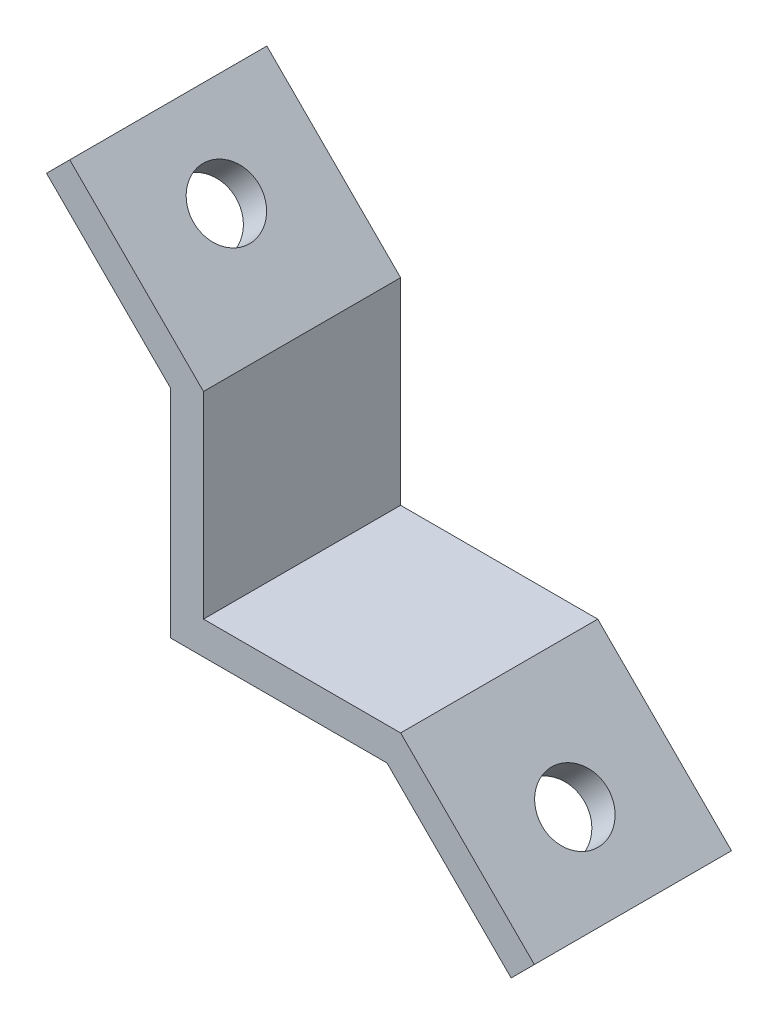
SolidWorks part; units mm, degrees
ref_plane "前视基准面" through (0, 0, 0) normal (0, 0, 1) x (1, 0, 0)
ref_plane "上视基准面" through (0, 0, 0) normal (0, 1, 0) x (1, 0, 0)
ref_plane "右视基准面" through (0, 0, 0) normal (1, 0, 0) x (0, 0, -1)
sketch "草图1" plane through (0, 0, 0) normal (0, 0, 1) x (1, 0, 0)
  line L0 (0, 0) -> (0, 60)
  line L1 (0, 60) -> (-10, 60)
  line L2 (-10, 60) -> (-10, -10)
  line L3 (-10, -10) -> (60, -10)
  line L4 (60, -10) -> (60, 0)
  line L5 (60, 0) -> (0, 0)
  dimension "D1" = 60
  dimension "D2" = 60
  dimension "D3" = 10
  dimension "D4" = 10
extrude "凸台-拉伸1" add sketch "草图1" along normal blind 60
sketch "草图2" plane through (0, 0, 0) normal (0, 0, 1) x (1, 0, 0)
  line L0 (0, 60) -> (-40.7107, 100.7107)
  line L1 (-40.7107, 100.7107) -> (-47.7817, 93.6396)
  line L2 (-47.7817, 93.6396) -> (-10, 55.8579)
  line L4 (-10, 55.8579) -> (-10, 60)
  line L5 (-10, 60) -> (0, 60)
  line L6 (60, 0) -> (100.7107, -40.7107)
  line L7 (100.7107, -40.7107) -> (93.6396, -47.7817)
  line L8 (93.6396, -47.7817) -> (55.8579, -10)
  line L10 (55.8579, -10) -> (60, -10)
  line L11 (60, -10) -> (60, 0)
extrude "凸台-拉伸2" add sketch "草图2" along normal blind 60
sketch "草图3" plane through (22.9289, 22.9289, 0) normal (-0.7071, -0.7071, 0) x (0, 0, 1)
  line L0 (60, -100) -> (0, -100) construction
  line L1 (60, 100) -> (0, 100) construction
  circle A0 centre (30, 75) radius 10
  circle A1 centre (30, -75) radius 10
  dimension "D1" = 25
  dimension "D2" = 25
extrude "切除-拉伸1" cut sketch "草图3" against normal blind 60
